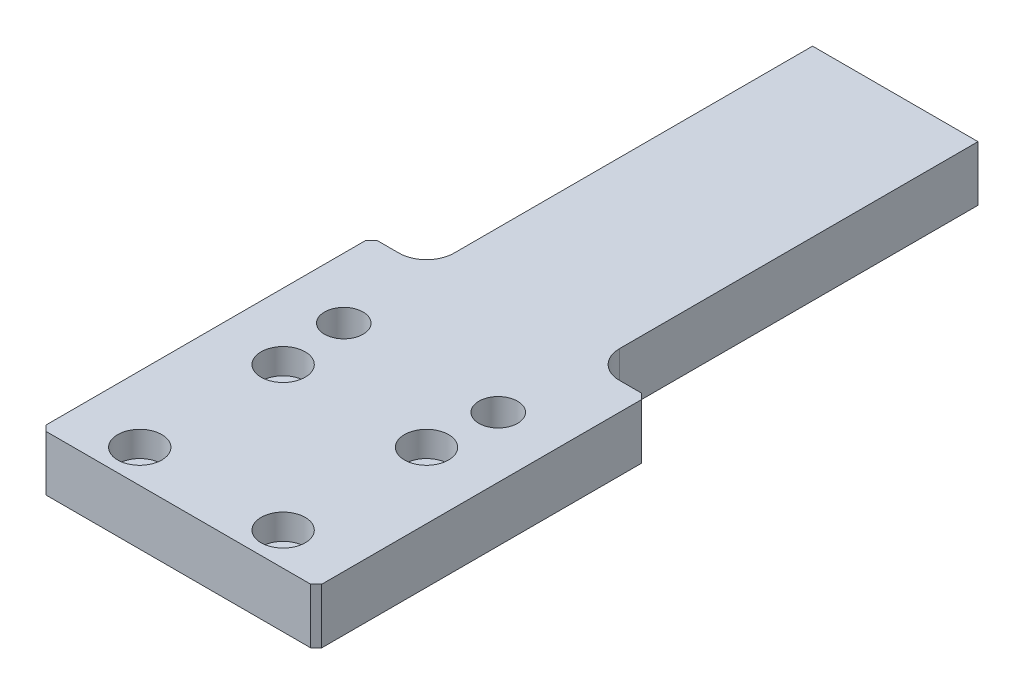
from build123d import *

# Parameters (mm, degrees)
SKETCH_1_W                = 50
SKETCH_1_H                = 60
EXTRUDE_1_DEPTH           = 5
HOLE_WIZARD_1_D           = 4.5
HOLE_WIZARD_1_CBORE_D     = 8
HOLE_WIZARD_1_CBORE_DEPTH = 4.6
M8X1_0_1_D                = 7
SKETCH_8_W                = 30
SKETCH_8_H                = 70
EXTRUDE_2_DEPTH           = 10
CHAMFER_1_SIZE            = 1
FILLET_1_R                = 5
HOLE_WIZARD_M4_1_D        = 3.3
HOLE_WIZARD_M4_1_DEPTH    = 10.1
HOLE_WIZARD_M4_1_TIP      = 0.991420021


with BuildPart() as part:
    # 草图1 → 凸台-拉伸1 (new, symmetric)
    with BuildSketch(Plane(origin=(0, 0, 0), x_dir=(1, 0, 0), z_dir=(0, 1, 0))):
        Rectangle(SKETCH_1_W, SKETCH_1_H)
    extrude(amount=EXTRUDE_1_DEPTH, both=True)

    # 打孔尺寸(%根据)内六角圆柱头螺钉的类型1 (through all)
    with Locations(Plane(origin=(0, 5, 0), x_dir=(1, 0, 0), z_dir=(0, 1, 0))):
        with Locations((13, -24), (13, 2), (-13, 2), (-13, -24)):
            CounterBoreHole(HOLE_WIZARD_1_D / 2, HOLE_WIZARD_1_CBORE_D / 2, HOLE_WIZARD_1_CBORE_DEPTH)

    # M8x1.0 螺纹孔1 (through all)
    with Locations(Plane(origin=(0, 5, 0), x_dir=(1, 0, 0), z_dir=(0, 1, 0))):
        with Locations((-14, 14), (14, 14)):
            Hole(M8X1_0_1_D / 2)

    # 草图8 → 凸台-拉伸2 (add)
    with BuildSketch(Plane(origin=(0, 5, 0), x_dir=(1, 0, 0), z_dir=(0, 1, 0))):
        with Locations((0, 65)):
            Rectangle(SKETCH_8_W, SKETCH_8_H)
    extrude(amount=-EXTRUDE_2_DEPTH)

    # 倒角1
    chamfer_1_edges = [part.edges().sort_by_distance(p)[0] for p in [
        (25, 0, 30),
        (-25, 0, 30),
        (-25, 0, -30),
        (25, 0, -30),
    ]]
    chamfer(chamfer_1_edges, length=CHAMFER_1_SIZE)

    # 圆角1
    fillet_1_edges = [part.edges().sort_by_distance(p)[0] for p in [
        (-15, 0, -30),
        (15, 0, -30),
    ]]
    fillet(fillet_1_edges, radius=FILLET_1_R)

    # M4 螺纹孔1
    with Locations(Plane(origin=(0, 0, -100), x_dir=(-1, 0, 0), z_dir=(0, 0, -1))):
        with Locations((10, 0), (-10, 0)):
            Hole(HOLE_WIZARD_M4_1_D / 2, depth=HOLE_WIZARD_M4_1_DEPTH)
            with Locations((0, 0, -(HOLE_WIZARD_M4_1_DEPTH + HOLE_WIZARD_M4_1_TIP / 2))):  # 118° drill point
                Cone(0, HOLE_WIZARD_M4_1_D / 2, HOLE_WIZARD_M4_1_TIP, mode=Mode.SUBTRACT)


solid = part.part
